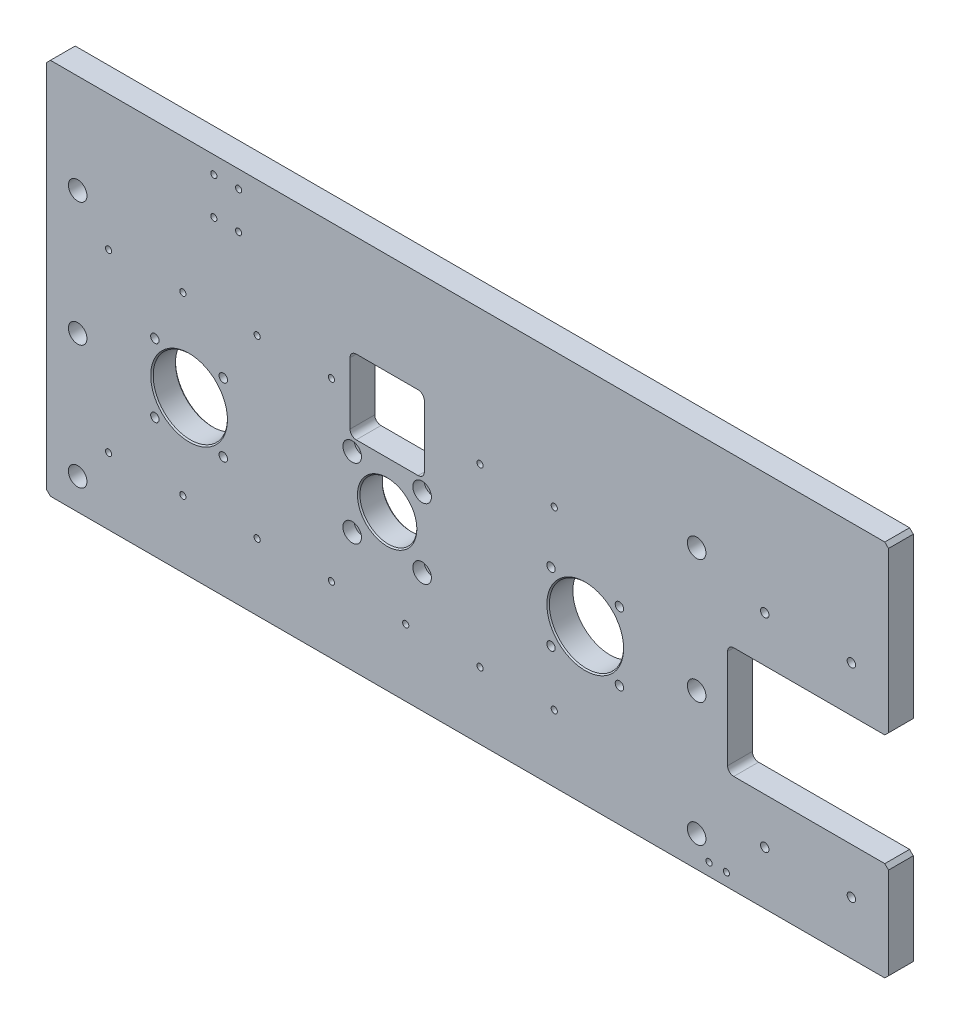
SolidWorks part; units mm, degrees
material "Q235-A"
ref_plane "Front Plane" through (0, 0, 0) normal (0, 0, 1) x (1, 0, 0)
ref_plane "Top Plane" through (0, 0, 0) normal (0, 1, 0) x (1, 0, 0)
ref_plane "Right Plane" through (0, 0, 0) normal (1, 0, 0) x (0, 0, -1)
sketch "Sketch1" plane through (0, 0, 0) normal (0, 0, 1) x (1, 0, 0)
  line L0 (421.7594, -47.943) -> (421.7594, -127.943)
  line L1 (-258.2406, 177.057) -> (421.7594, 177.057)
  line L2 (-258.2406, 177.057) -> (-258.2406, -127.943)
  line L3 (-258.2406, -127.943) -> (421.7594, -127.943)
  line L4 (421.7594, 177.057) -> (421.7594, 42.057)
  line L5 (421.7594, -47.943) -> (291.7594, -47.943)
  line L7 (421.7594, 42.057) -> (291.7594, 42.057)
  line L8 (291.7594, -47.943) -> (291.7594, 42.057)
  line L10 (-13.2406, 95.057) -> (46.7594, 95.057)
  line L11 (-13.2406, 95.057) -> (-13.2406, 35.057)
  line L12 (-13.2406, 35.057) -> (46.7594, 35.057)
  line L13 (46.7594, 95.057) -> (46.7594, 35.057)
  dimension "D1" = 680
  dimension "D2" = 305
  dimension "D3" = 130
  dimension "D4" = 90
  dimension "D5" = 80
  dimension "D6" = 60
  dimension "D7" = 60
  dimension "D8" = 163
  dimension "D9" = 245
extrude "Boss-Extrude1" add sketch "Sketch1" along normal blind 20
fillet "Fillet1" radius 5 6 edges at (291.7594, -47.943, 10) (291.7594, 42.057, 10) (46.7594, 35.057, 10) (-13.2406, 35.057, 10) (46.7594, 95.057, 10) (-13.2406, 95.057, 10)
chamfer "Chamfer1" distance 3 angle 45 6 edges at (-258.2406, -127.943, 10) (-258.2406, 177.057, 10) (421.7594, 177.057, 10) (421.7594, 42.057, 10) (421.7594, -47.943, 10) (421.7594, -127.943, 10)
sketch "Sketch2" plane through (0, 0, 20) normal (0, 0, 1) x (1, 0, 0)
  line L0 (377.9652, -2.943) -> (-297.5193, -2.943) construction
  line L1 (-255.2406, -127.943) -> (418.7594, -127.943) construction
  line L2 (-258.2406, 174.057) -> (-258.2406, -124.943) construction
  circle A0 centre (-143.2406, -2.943) radius 30
  circle A1 centre (16.7594, -2.943) radius 23
  circle A2 centre (176.7594, -2.943) radius 30
  dimension "D2" = 320
  dimension "D3" = 160
  dimension "D4" = 275
  dimension "D5" = 60
  dimension "D6" = 46
  dimension "D7" = 60
  dimension "D1" = 125
extrude "Cut-Extrude1" cut sketch "Sketch2" against normal blind 20
chamfer "Chamfer2" distance 1 angle 45 5 edges at (206.7594, -2.943, 20) (-113.2406, -2.943, 0) (39.7594, -2.943, 0) (39.7594, -2.943, 20) (-113.2406, -2.943, 20)
sketch "Sketch3" plane through (0, 0, 20) normal (0, 0, 1) x (1, 0, 0)
  line L0 (-258.2406, 174.057) -> (-258.2406, -124.943) construction
  line L1 (-233.2406, 97.057) -> (266.7594, 97.057)
  line L2 (-233.2406, 97.057) -> (-233.2406, -102.943)
  line L3 (-233.2406, -102.943) -> (266.7594, -102.943)
  line L4 (266.7594, 97.057) -> (266.7594, -102.943)
  line L5 (-233.2406, -2.943) -> (266.7594, -2.943)
  line L6 (-255.2406, -127.943) -> (418.7594, -127.943) construction
  line L7 (-208.2406, -73.943) -> (-208.2406, 68.057)
  line L12 (-148.2406, -73.943) -> (-148.2406, 68.057)
  line L13 (-88.2406, -73.943) -> (-88.2406, 68.057)
  line L14 (-28.2406, -73.943) -> (-28.2406, 68.057)
  line L15 (31.7594, -73.943) -> (31.7594, 68.057)
  line L16 (91.7594, -73.943) -> (91.7594, 68.057)
  line L17 (151.7594, -73.943) -> (151.7594, 68.057)
  line L18 (276.7594, -117.943) -> (290.7594, -117.943)
  line L19 (321.7594, 79.057) -> (391.7594, 79.057)
  line L20 (321.7594, 79.057) -> (321.7594, -84.943)
  line L21 (321.7594, -84.943) -> (391.7594, -84.943)
  line L22 (391.7594, 79.057) -> (391.7594, -84.943)
  line L23 (-143.2406, -2.943) -> (-103.2406, 37.057)
  line L24 (-123.2406, 163.057) -> (-103.2406, 163.057)
  line L25 (-123.2406, 163.057) -> (-123.2406, 133.057)
  line L26 (-123.2406, 133.057) -> (-103.2406, 133.057)
  line L27 (-103.2406, 163.057) -> (-103.2406, 133.057)
  line L29 (-11.4906, -31.193) -> (45.0094, -31.193)
  line L30 (-11.4906, -31.193) -> (-11.4906, 25.307)
  line L31 (-11.4906, 25.307) -> (45.0094, 25.307)
  line L32 (45.0094, -31.193) -> (45.0094, 25.307)
  line L33 (-11.4906, -31.193) -> (45.0094, 25.307) construction
  line L34 (-11.4906, 25.307) -> (45.0094, -31.193) construction
  circle A0 centre (-143.2406, -2.943) radius 39
  circle A1 centre (-115.6099, 24.6876) radius 3.3852
  circle A2 centre (-115.6099, -30.5737) radius 3.3852
  circle A3 centre (-170.8713, -30.5737) radius 3.3852
  circle A4 centre (-170.8713, 24.6876) radius 3.3852
  circle A5 centre (149.1287, 24.6876) radius 3.3852
  circle A6 centre (204.3901, 24.6876) radius 3.3852
  circle A7 centre (204.3901, -30.5737) radius 3.3852
  circle A8 centre (149.1287, -30.5737) radius 3.3852
  point P13 (-208.2406, -2.943)
  point P50 (-143.2406, -2.943)
  point P56 (16.7594, -2.943)
  dimension "D18" = 4
  dimension "D1" = 500
  dimension "D2" = 25
  dimension "D3" = 200
  dimension "D4" = 25
  dimension "D5" = 142
  dimension "D6" = 50
  dimension "D7" = 43
  dimension "D8" = 164
  dimension "D9" = 70
  dimension "D10" = 580
  dimension "D11" = 14
  dimension "D12" = 10
  dimension "D13" = 535
  dimension "D14" = 20
  dimension "D15" = 30
  dimension "D16" = 135
  dimension "D17" = 261
  dimension "D19" = 56.5
  dimension "D20" = 56.5
hole_wizard "M8 Tapped Hole1" positions "Sketch4" profile "Sketch5" tap size "M8" standard "GB" end condition through all
sketch "Sketch4" plane through (0, 0, 20) normal (0, 0, 1) x (1, 0, 0)
  point P0 (321.7594, 79.057)
  point P3 (391.7594, 79.057)
  point P6 (391.7594, -84.943)
  point P9 (321.7594, -84.943)
cosmetic thread "Cosmetic thread 1" parameters "D2"=8
cosmetic thread "Cosmetic thread 2" parameters "D2"=8
cosmetic thread "Cosmetic thread 3" parameters "D2"=8
cosmetic thread "Cosmetic thread 4" parameters "D2"=8
sketch "Sketch5" plane through (321.7594, 79.057, 20) normal (1, 0, 0) x (0, -1, 0)
  line L0 (0, 0) -> (0, 20)
  line L1 (0, 20) -> (3.4, 20)
  line L2 (3.4, 20) -> (3.4, 0)
  line L5 (3.4, 0) -> (0, 0)
  line L11 (0, -6.35) -> (0, 107.95) construction
  dimension "通孔螺纹孔钻头直径" = 6.8
  dimension "通孔螺纹孔钻头深度" = 20
hole_wizard "M6 Tapped Hole1" positions "Sketch6" profile "Sketch7" tap size "M6" standard "GB" end condition through all
sketch "Sketch6" plane through (0, 0, 20) normal (0, 0, 1) x (1, 0, 0)
  point P0 (276.7594, -117.943)
  point P3 (290.7594, -117.943)
cosmetic thread "Cosmetic thread 5" parameters "D2"=6
cosmetic thread "Cosmetic thread 6" parameters "D2"=6
sketch "Sketch7" plane through (276.7594, -117.943, 20) normal (1, 0, 0) x (0, -1, 0)
  line L0 (0, 0) -> (0, 20)
  line L1 (0, 20) -> (2.5, 20)
  line L2 (2.5, 20) -> (2.5, 0)
  line L5 (2.5, 0) -> (0, 0)
  line L11 (0, -6.35) -> (0, 107.95) construction
  dimension "通孔螺纹孔钻头直径" = 5
  dimension "通孔螺纹孔钻头深度" = 20
hole_wizard "M6 Tapped Hole2" positions "Sketch8" profile "Sketch9" tap size "M6" standard "GB"
sketch "Sketch8" plane through (0, 0, 20) normal (0, 0, 1) x (1, 0, 0)
  point P0 (-208.2406, 68.057)
  point P3 (-208.2406, -73.943)
  point P6 (-148.2406, -73.943)
  point P9 (-88.2406, -73.943)
  point P12 (-88.2406, 68.057)
  point P15 (-148.2406, 68.057)
  point P18 (-28.2406, 68.057)
  point P21 (-28.2406, -73.943)
  point P24 (31.7594, -73.943)
  point P27 (91.7594, -73.943)
  point P30 (151.7594, -73.943)
  point P33 (151.7594, 68.057)
  point P36 (91.7594, 68.057)
sketch "Sketch9" plane through (-208.2406, 68.057, 20) normal (1, 0, 0) x (0, -1, 0)
  line L0 (0, 0) -> (0, 14.5022)
  line L1 (0, 14.5022) -> (2.5, 13)
  line L2 (2.5, 13) -> (2.5, 0)
  line L5 (2.5, 0) -> (0, 0)
  line L10 (0, 14.5022) -> (-2.5, 13) construction
  line L11 (0, -6.35) -> (0, 107.95) construction
  dimension "螺纹孔钻头直径" = 5
  dimension "螺纹孔钻头深度" = 13
  dimension "导头角度" = 118
cosmetic thread "Cosmetic thread 7" parameters "D1"=12, "D2"=6
cosmetic thread "Cosmetic thread 8" parameters "D1"=12, "D2"=6
cosmetic thread "Cosmetic thread 9" parameters "D1"=12, "D2"=6
cosmetic thread "Cosmetic thread 10" parameters "D1"=12, "D2"=6
cosmetic thread "Cosmetic thread 11" parameters "D1"=12, "D2"=6
cosmetic thread "Cosmetic thread 12" parameters "D1"=12, "D2"=6
cosmetic thread "Cosmetic thread 13" parameters "D1"=12, "D2"=6
cosmetic thread "Cosmetic thread 14" parameters "D1"=12, "D2"=6
cosmetic thread "Cosmetic thread 15" parameters "D1"=12, "D2"=6
cosmetic thread "Cosmetic thread 16" parameters "D1"=12, "D2"=6
cosmetic thread "Cosmetic thread 17" parameters "D1"=12, "D2"=6
cosmetic thread "Cosmetic thread 18" parameters "D1"=12, "D2"=6
cosmetic thread "Cosmetic thread 19" parameters "D1"=12, "D2"=6
hole_wizard "M8 Tapped Hole2" positions "Sketch10" profile "Sketch11" tap size "M8" standard "GB" end condition through all
sketch "Sketch10" plane through (0, 0, 20) normal (0, 0, 1) x (1, 0, 0)
  point P0 (-170.8713, 24.6876)
  point P3 (-170.8713, -30.5737)
  point P6 (-115.6099, -30.5737)
  point P9 (-115.6099, 24.6876)
  point P12 (149.1287, 24.6876)
  point P15 (204.3901, 24.6876)
  point P18 (204.3901, -30.5737)
  point P21 (149.1287, -30.5737)
sketch "Sketch11" plane through (-170.8713, 24.6876, 20) normal (1, 0, 0) x (0, -1, 0)
  line L0 (0, 0) -> (0, 20)
  line L1 (0, 20) -> (3.4, 20)
  line L2 (3.4, 20) -> (3.4, 0)
  line L5 (3.4, 0) -> (0, 0)
  line L11 (0, -6.35) -> (0, 107.95) construction
  dimension "通孔螺纹孔钻头直径" = 6.8
  dimension "通孔螺纹孔钻头深度" = 20
cosmetic thread "Cosmetic thread 20" parameters "D2"=8
cosmetic thread "Cosmetic thread 21" parameters "D2"=8
cosmetic thread "Cosmetic thread 22" parameters "D2"=8
cosmetic thread "Cosmetic thread 23" parameters "D2"=8
cosmetic thread "Cosmetic thread 24" parameters "D2"=8
cosmetic thread "Cosmetic thread 25" parameters "D2"=8
cosmetic thread "Cosmetic thread 26" parameters "D2"=8
cosmetic thread "Cosmetic thread 27" parameters "D2"=8
hole_wizard "M6 Tapped Hole3" positions "Sketch12" profile "Sketch13" tap size "M6" standard "GB" end condition through all
sketch "Sketch12" plane through (0, 0, 20) normal (0, 0, 1) x (1, 0, 0)
  point P0 (-123.2406, 163.057)
  point P3 (-103.2406, 163.057)
  point P6 (-103.2406, 133.057)
  point P9 (-123.2406, 133.057)
sketch "Sketch13" plane through (-123.2406, 163.057, 20) normal (1, 0, 0) x (0, -1, 0)
  line L0 (0, 0) -> (0, 20)
  line L1 (0, 20) -> (2.5, 20)
  line L2 (2.5, 20) -> (2.5, 0)
  line L5 (2.5, 0) -> (0, 0)
  line L11 (0, -6.35) -> (0, 107.95) construction
  dimension "通孔螺纹孔钻头直径" = 5
  dimension "通孔螺纹孔钻头深度" = 20
cosmetic thread "Cosmetic thread 28" parameters "D2"=6
cosmetic thread "Cosmetic thread 29" parameters "D2"=6
cosmetic thread "Cosmetic thread 30" parameters "D2"=6
cosmetic thread "Cosmetic thread 31" parameters "D2"=6
hole_wizard "Hole1" positions "Sketch14" profile "Sketch15" legacy end condition through all
sketch "Sketch14" plane through (0, 0, 20) normal (0, 0, 1) x (1, 0, 0)
  point P0 (-233.2406, 97.057)
  point P3 (-233.2406, -2.943)
  point P6 (-233.2406, -102.943)
  point P9 (266.7594, 97.057)
  point P12 (266.7594, -102.943)
  point P15 (266.7594, -2.943)
sketch "Sketch15" plane through (-233.2406, 97.057, 20) normal (1, 0, 0) x (0, -1, 0)
  line L0 (0, 0) -> (0, 20)
  line L1 (0, 20) -> (4.5, 20)
  line L2 (4.5, 20) -> (4.5, 11)
  line L3 (4.5, 11) -> (7.5, 11)
  line L4 (7.5, 11) -> (7.5, 0)
  line L5 (7.5, 0) -> (0, 0)
  line L6 (0, 110) -> (0, -10) construction
  dimension "直径" = 9
  dimension "深度" = 20
  dimension "柱坑直径" = 15
  dimension "柱坑深度" = 11
hole_wizard "Hole2" positions "Sketch16" profile "Sketch17" legacy end condition through all
sketch "Sketch16" plane through (0, 0, 20) normal (0, 0, 1) x (1, 0, 0)
  point P0 (-11.4906, 25.307)
  point P3 (45.0094, 25.307)
  point P6 (45.0094, -31.193)
  point P9 (-11.4906, -31.193)
sketch "Sketch17" plane through (-11.4906, 25.307, 20) normal (1, 0, 0) x (0, -1, 0)
  line L0 (0, 0) -> (0, 20)
  line L1 (0, 20) -> (4.5, 20)
  line L2 (4.5, 20) -> (4.5, 9)
  line L3 (4.5, 9) -> (7.5, 9)
  line L4 (7.5, 9) -> (7.5, 0)
  line L5 (7.5, 0) -> (0, 0)
  line L6 (0, 110) -> (0, -10) construction
  dimension "直径" = 9
  dimension "深度" = 20
  dimension "柱坑直径" = 15
  dimension "柱坑深度" = 9
